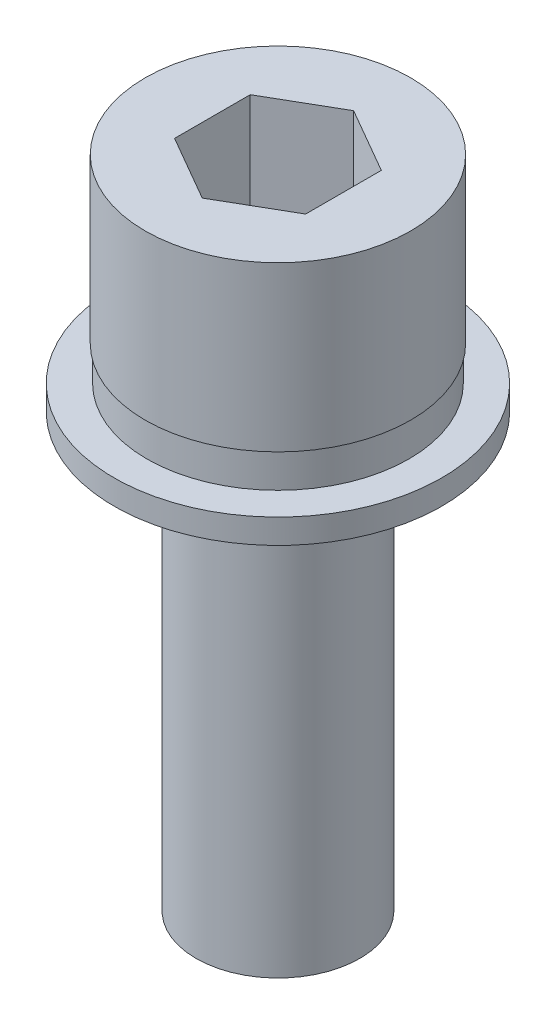
SolidWorks part; units mm, degrees
ref_plane "Front Plane" through (0, 0, 0) normal (0, 0, 1) x (1, 0, 0)
ref_plane "Top Plane" through (0, 0, 0) normal (0, 1, 0) x (1, 0, 0)
ref_plane "Right Plane" through (0, 0, 0) normal (1, 0, 0) x (0, 0, -1)
sketch "Sketch 1" plane through (0, 0, 0) normal (0, 0, 1) x (1, 0, 0)
  line L0 (0, 11.322) -> (0, -25.8305) construction
  line L1 (-9.8983, 0) -> (13.1525, 0) construction
  line L2 (0, 10) -> (-8.1, 10)
  line L3 (-8.1, 10) -> (-8.1, 0)
  line L4 (-8.1, 0) -> (-5, 0)
  line L5 (-5, 0) -> (-5, -30)
  line L6 (-5, -30) -> (0, -30)
  line L7 (0, -30) -> (0, 10)
  dimension "D1" = 10
  dimension "D2" = 30
  dimension "D3" = 10
  dimension "D4" = 16.2
revolve "Revolve 1" add sketch "Sketch 1" angle 360 about L0
sketch "Sketch 2" plane through (0, 10, 0) normal (0, 1, 0) x (1, 0, 0)
  line L1 (0, 4.6188) -> (-4, 2.3094)
  line L2 (-4, 2.3094) -> (-4, -2.3094)
  line L3 (-4, -2.3094) -> (0, -4.6188)
  line L4 (0, -4.6188) -> (4, -2.3094)
  line L5 (4, -2.3094) -> (4, 2.3094)
  line L6 (4, 2.3094) -> (0, 4.6188)
  circle A0 centre (0, 0) radius 4 construction
  dimension "D1" = 8
extrude "Cut-Extrude 1" cut sketch "Sketch 2" against normal blind 6
sketch "Sketch 3" plane through (0, 0, 0) normal (0, -1, 0) x (1, 0, 0)
  circle A0 centre (0, 0) radius 5
  circle A1 centre (0, 0) radius 8
  dimension "D1" = 3
  dimension "D2" = 10
extrude "Boss-Extrude 1" add sketch "Sketch 3" along normal blind 2.1 separate body
sketch "Sketch 4" plane through (0, -2.1, 0) normal (0, -1, 0) x (1, 0, 0)
  circle A0 centre (0, 0) radius 10
  circle A1 centre (0, 0) radius 5
  dimension "D1" = 10
  dimension "D2" = 20
extrude "Boss-Extrude 2" add sketch "Sketch 4" along normal blind 1.5 separate body
